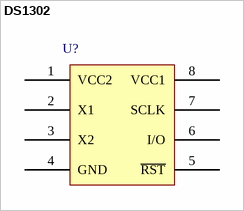
[diagram p0: symbol DS1302]
# Altium schematic symbol library MISC82171.SchLib: 1 symbol
Pins are listed as number, name and electrical type; pins without a type are passive.


## DS1302
designator U?
footprint DIP8
pins: 1 VCC2, 2 X1, 3 X2, 4 GND, 5 ~{RST}, 6 I/O, 7 SCLK, 8 VCC1